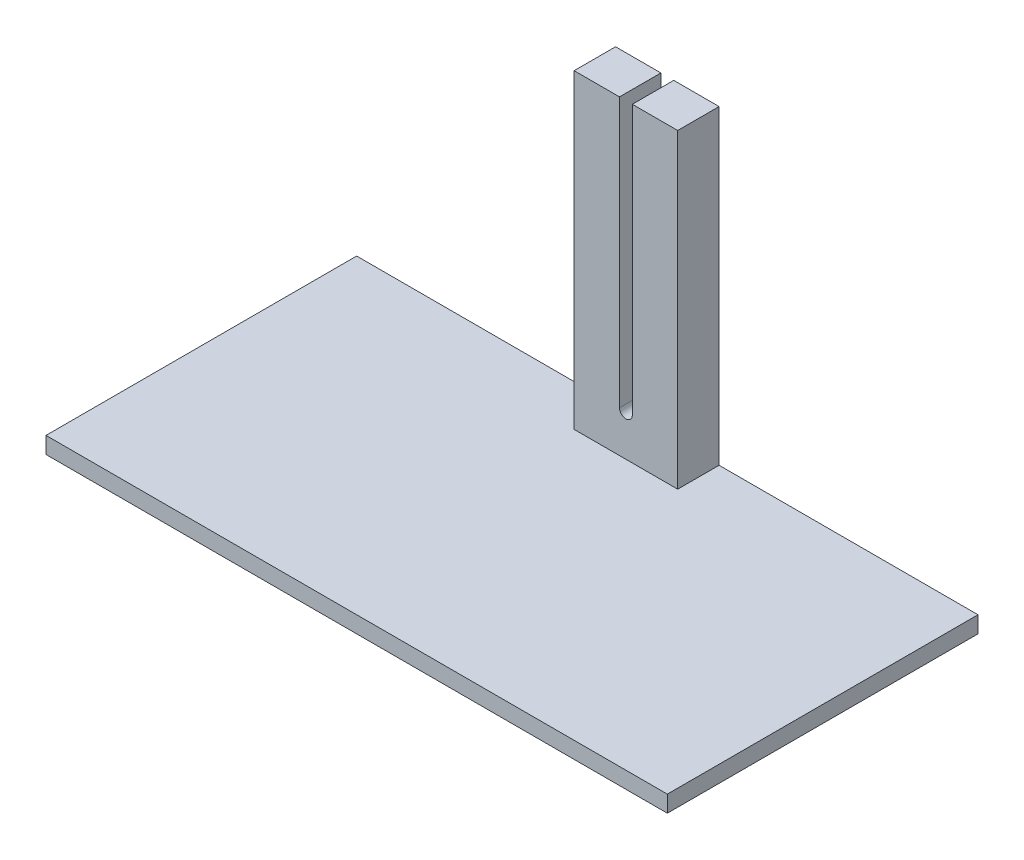
from build123d import *

# Parameters (mm, degrees)
SKETCH1_W           = 300
SKETCH1_H           = 150
BOSS_EXTRUDE1_DEPTH = 8
SKETCH2_W           = 50
SKETCH2_H           = 20
BOSS_EXTRUDE2_DEPTH = 150
CUT_EXTRUDE1_DEPTH  = 254.700610957


with BuildPart() as part:
    # Sketch1 → Boss-Extrude1 (new body)
    with BuildSketch(Plane(origin=(0, 0, 0), x_dir=(1, 0, 0), z_dir=(0, 1, 0))):
        Rectangle(SKETCH1_W, SKETCH1_H)
    extrude(amount=BOSS_EXTRUDE1_DEPTH)

    # Sketch2 → Boss-Extrude2 (add)
    with BuildSketch(Plane(origin=(0, 8, 0), x_dir=(1, 0, 0), z_dir=(0, 1, 0))):
        with Locations((0, 65)):
            Rectangle(SKETCH2_W, SKETCH2_H)
    extrude(amount=BOSS_EXTRUDE2_DEPTH)

    # Sketch3 → Cut-Extrude1 (cut, through all)
    with BuildSketch(Plane.XY.offset(-55)):
        with BuildLine():
            Line((3.1, 158), (3.1, 28))
            ThreePointArc((3.1, 28), (0, 24.9), (-3.1, 28))
            Line((-3.1, 28), (-3.1, 158))
            ThreePointArc((-3.1, 158), (0, 161.1), (3.1, 158))
        make_face()
    extrude(amount=-CUT_EXTRUDE1_DEPTH, mode=Mode.SUBTRACT)


solid = part.part
